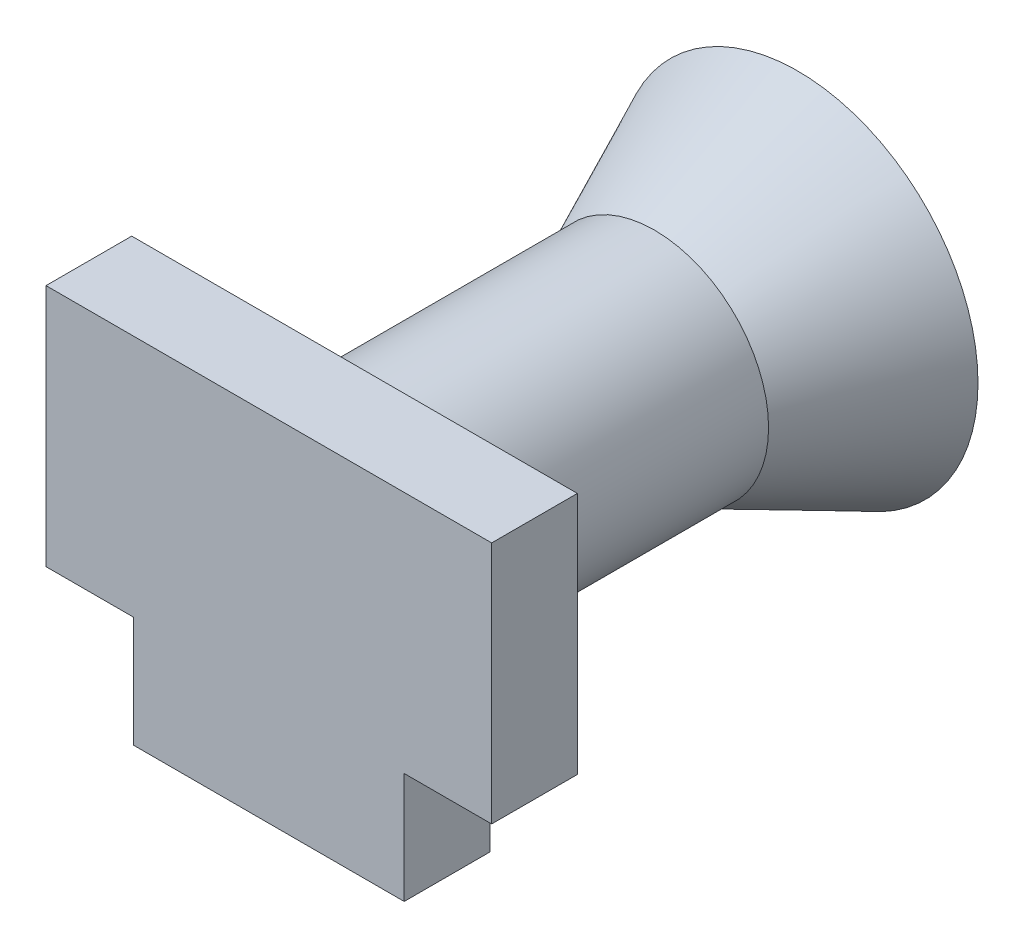
SolidWorks part; units mm, degrees
ref_plane "Front Plane" through (0, 0, 0) normal (0, 0, 1) x (1, 0, 0)
ref_plane "Top Plane" through (0, 0, 0) normal (0, 1, 0) x (1, 0, 0)
ref_plane "Right Plane" through (0, 0, 0) normal (1, 0, 0) x (0, 0, -1)
sketch "Sketch1" plane through (0, 0, 0) normal (0, 0, 1) x (1, 0, 0)
  line L0 (0, 47.0939) -> (0, -43.557) construction
  line L1 (15.792, 0) -> (-15.792, 0)
  line L2 (-15.792, 0) -> (-15.792, 12.9327)
  line L3 (-15.792, 12.9327) -> (-25.996, 12.9327)
  line L4 (-25.996, 12.9327) -> (-25.996, 41.33)
  line L5 (-25.996, 41.33) -> (25.996, 41.33)
  line L6 (15.792, 0) -> (15.792, 12.9327)
  line L7 (15.792, 12.9327) -> (25.996, 12.9327)
  line L8 (25.996, 12.9327) -> (25.996, 41.33)
  point P14 (0, 0)
  point P17 (0, 41.33)
  dimension "D1" = 41.33
extrude "Boss-Extrude1" add sketch "Sketch1" against normal blind 10
sketch "Sketch2" plane through (0, 0, -10) normal (0, 0, -1) x (-1, 0, 0)
  circle A0 centre (0, 24.131) radius 13.3007
extrude "Boss-Extrude2" add sketch "Sketch2" along normal blind 35
sketch "Sketch5" plane through (0, 0, 0) normal (1, 0, 0) x (0, 0, -1)
  line L0 (45, 24.131) -> (64.6558, 24.131) construction
  line L1 (45, 10.8303) -> (45, 37.4317) construction
  line L2 (45, 37.4317) -> (61.7117, 45.1518)
  line L3 (61.7117, 45.1518) -> (61.7117, 24.131)
  line L4 (61.7117, 24.131) -> (45, 24.131)
  line L5 (45, 24.131) -> (45, 37.4317)
revolve "Revolve4" add sketch "Sketch5" angle 360 about L0
